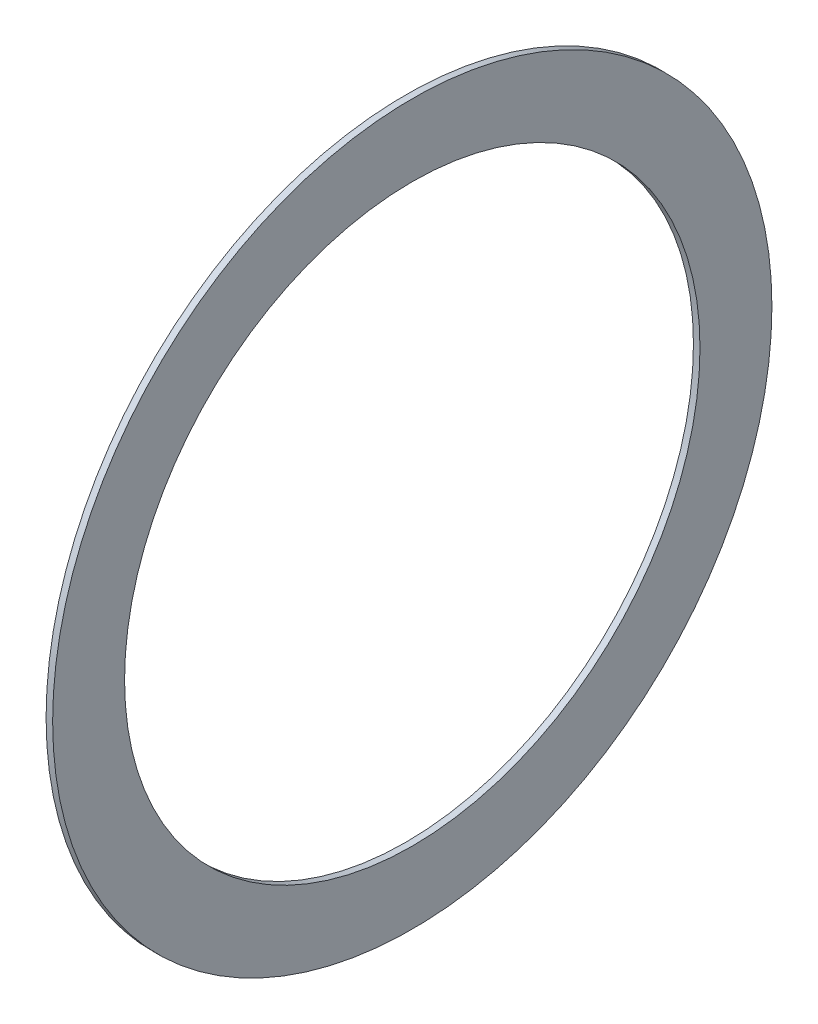
SolidWorks part; units mm, degrees
material "XB150"
ref_plane "前视基准面" through (0, 0, 0) normal (0, 0, 1) x (1, 0, 0)
ref_plane "上视基准面" through (0, 0, 0) normal (0, 1, 0) x (1, 0, 0)
ref_plane "右视基准面" through (0, 0, 0) normal (1, 0, 0) x (0, 0, -1)
sketch "草图1" plane through (0, 0, 0) normal (1, 0, 0) x (0, 0, -1)
  circle A0 centre (0, 0) radius 22.5
  circle A1 centre (0, 0) radius 18
extrude "凸台-拉伸1" add sketch "草图1" along normal blind 0.41
